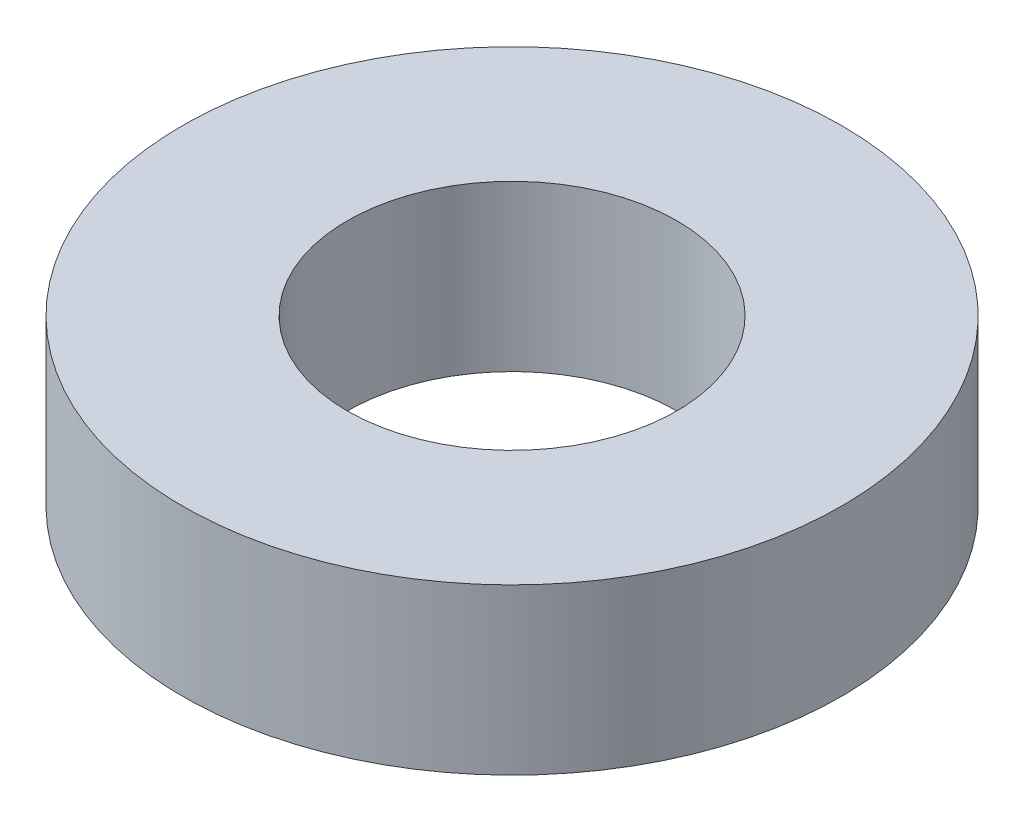
from build123d import *

# Parameters (mm, degrees)
SKETCH_1_W = 4
SKETCH_1_H = 4


with BuildPart() as part:
    # 草图1 → 旋转1 (revolve)
    with BuildSketch(Plane.XY, mode=Mode.PRIVATE) as revolve_1_sk:
        with Locations((6, -0.900336073)):
            Rectangle(SKETCH_1_W, SKETCH_1_H)
    revolve(revolve_1_sk.sketch.rotate(Axis((0, 0, 0), (0, 1, 0)), 90), axis=Axis((0, 0, 0), (0, 1, 0)))


solid = part.part
